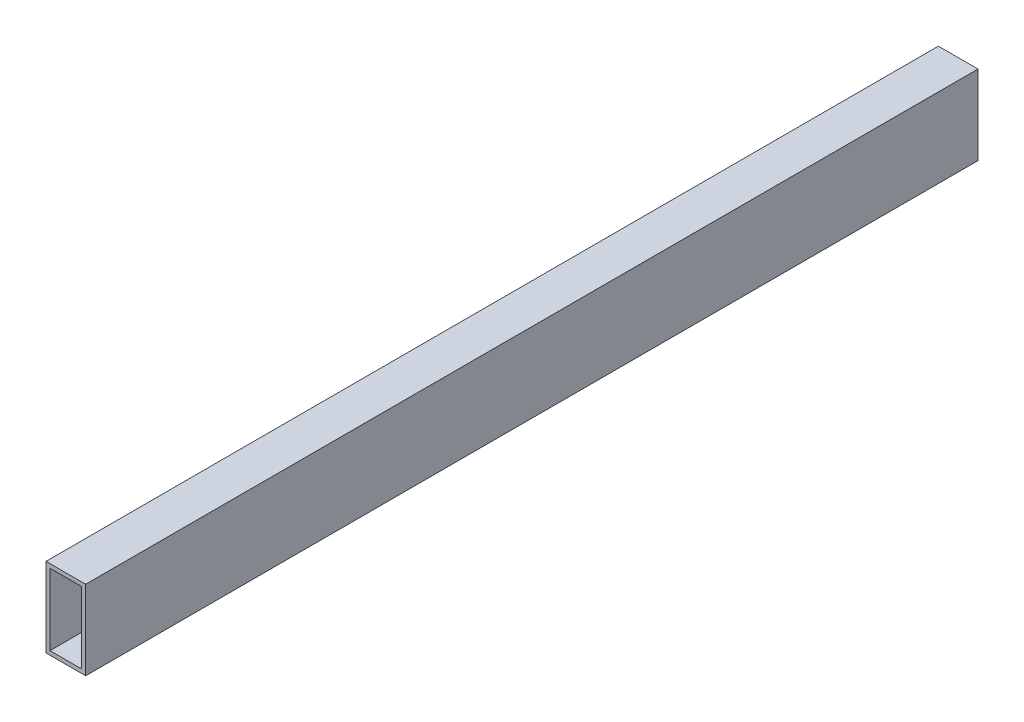
from build123d import *

# Parameters (mm, degrees)
SKETCH_1_W      = 40
SKETCH_1_H      = 80
SKETCH_1_W_2    = 32
SKETCH_1_H_2    = 72
EXTRUDE_1_DEPTH = 450


with BuildPart() as part:
    # 草图1 → 凸台-拉伸1 (new, symmetric)
    with BuildSketch(Plane.XY):
        Rectangle(SKETCH_1_W, SKETCH_1_H)
        Rectangle(SKETCH_1_W_2, SKETCH_1_H_2, mode=Mode.SUBTRACT)
    extrude(amount=EXTRUDE_1_DEPTH, both=True)


solid = part.part
